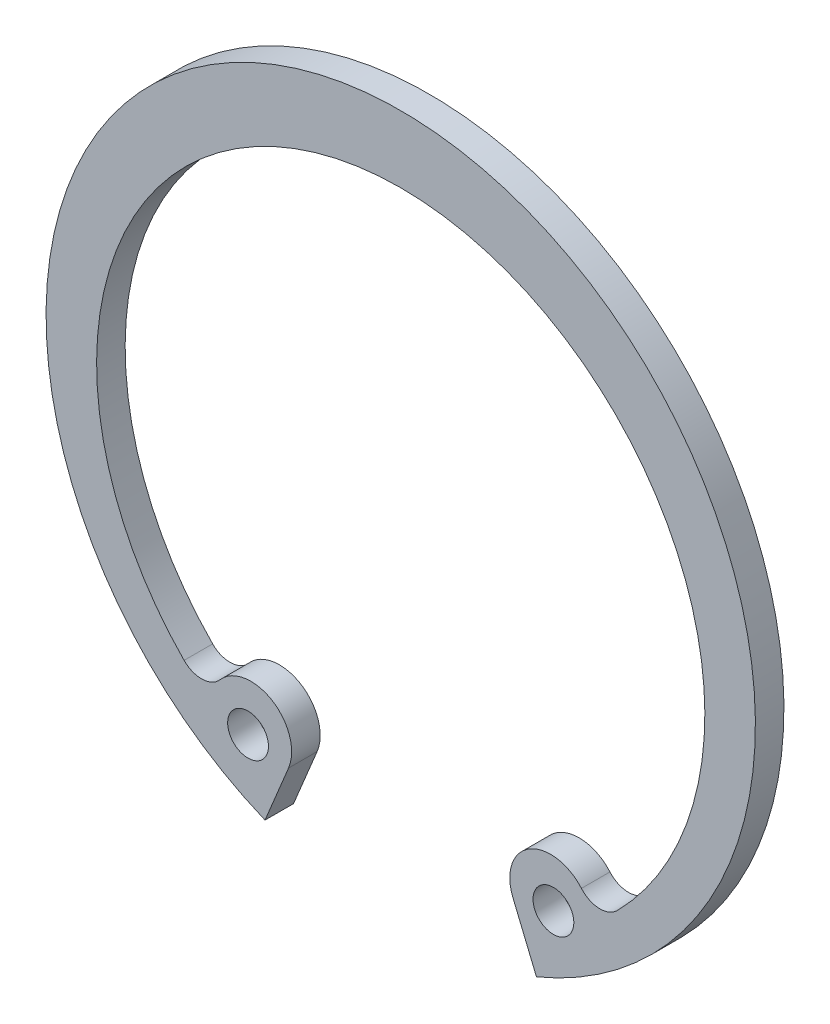
SolidWorks part; units mm, degrees
material "Q235"
ref_plane "Front" through (0, 0, 0) normal (0, 0, 1) x (1, 0, 0)
ref_plane "Top" through (0, 0, 0) normal (0, 1, 0) x (1, 0, 0)
ref_plane "Right" through (0, 0, 0) normal (1, 0, 0) x (0, 0, -1)
sketch "Dimension sketch" plane through (0, 0, 0) normal (0, 0, 1) x (1, 0, 0)
  line L0 (-21.75, 0) -> (21.75, 0) construction
  line L1 (0, 0) -> (-18.8361, -10.875) construction
  circle A0 centre (0, 0) radius 21.75
  point P5 (-15.55, 0)
  point P6 (2.5, 0)
  point P7 (2.5, 0)
  point P8 (4, 0)
  point P10 (-3.3, 0)
  point P11 (-1, 0)
  point P12 (-5.8, 0)
  point P13 (-17.3, 0)
  point P14 (20.1351, 11.625)
  dimension "d3" = 43.5
  dimension "d" = 37.3
  dimension "R1" = 2.5
  dimension "R2" = 1.5
  dimension "aa" = 45
  dimension "a" = 5.8
  dimension "d5" = 2.5
  dimension "c" = 1
  dimension "s" = 1.75
  dimension "m" = 30
sketch "Sketch1" plane through (0, 0, 0) normal (0, 0, 1) x (1, 0, 0)
  line L0 (0, 21.75) -> (0, -20.0944) construction
  line L1 (-6.8795, -16.6086) -> (-8.3234, -20.0944)
  line L2 (-9.5368, -16.4912) -> (-9.1892, -15.6519) construction
  line L3 (0, 0) -> (-8.3234, -20.0944) construction
  line L4 (6.8795, -16.6086) -> (8.3234, -20.0944)
  arc A0 (8.3234, -20.0944) -> (-8.3234, -20.0944) centre (0, 0) ccw
  arc A1 (13.2846, -14.0898) -> (-13.2846, -14.0898) centre (0, -1) ccw
  circle A2 centre (-9.363, -16.0715) radius 1.25
  arc A3 (-6.8795, -16.6086) -> (-11.081, -14.0176) centre (-9.1892, -15.6519) ccw
  arc A4 (-11.081, -14.0176) -> (-13.2846, -14.0898) centre (-12.2161, -13.037) cw
  circle A5 centre (9.363, -16.0715) radius 1.25
  arc A6 (6.8795, -16.6086) -> (11.081, -14.0176) centre (9.1892, -15.6519) cw
  arc A7 (11.081, -14.0176) -> (13.2846, -14.0898) centre (12.2161, -13.037) ccw
  dimension "D1" = 43.5
  dimension "D2" = 37.3
  dimension "D5" = 2.5
  dimension "D7" = 2.5
  dimension "D8" = 1.5
  dimension "D9" = 6.1
  dimension "D3" = 1
  dimension "D4" = 22.5
  dimension "D6" = 18.6
extrude "Base-Extrude" add sketch "Sketch1" along normal blind 1.75
